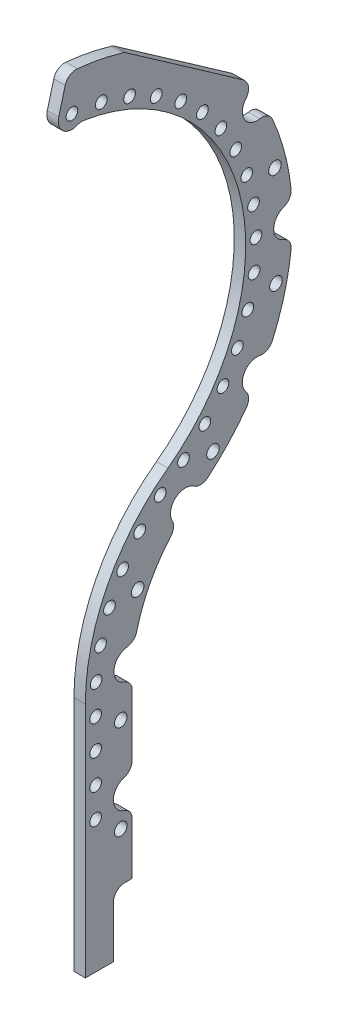
from build123d import *

# Parameters (mm, degrees)
SKETCH_3_R      = 1.025
SKETCH_3_R_2    = 1.1
EXTRUDE_1_DEPTH = 1
FILLET_R2_1_R   = 2


with BuildPart() as part:
    # 草图3 → 凸台-拉伸1 (new, symmetric)
    with BuildSketch(Plane(origin=(0, 0, 0), x_dir=(0, 0, -1), z_dir=(1, 0, 0))):
        with BuildLine():
            Line((17.7, -14.496003195), (17.7, -0.091005487))
            ThreePointArc((17.7, -0.091005487), (14.516449024, 2.667043271), (18.130694373, 4.830156842))
            ThreePointArc((18.130694373, 4.830156842), (20.784604254, 12.605737141), (25.63176658, 19.239582485))
            ThreePointArc((25.63176658, 19.239582485), (25.323964311, 23.435289305), (29.409373215, 22.431231514))
            ThreePointArc((29.409373215, 22.431231514), (34.557047376, 27.097753162), (38.858437765, 32.554218527))
            ThreePointArc((38.858437765, 32.554218527), (37.328835208, 36.351942354), (41.382561796, 36.926129595))
            ThreePointArc((41.382561796, 36.926129595), (44.352566659, 44.759188173), (45.696996288, 53.027818322))
            ThreePointArc((45.696996288, 53.027818322), (42.473459702, 55.551942354), (45.696996288, 58.076066385))
            ThreePointArc((45.696996288, 58.076066385), (44.352566659, 66.344696534), (41.382561796, 74.177755113))
            ThreePointArc((41.382561796, 74.177755113), (37.328835208, 74.751942354), (38.858437765, 78.54966618))
            ThreePointArc((38.858437765, 78.54966618), (38.104416138, 79.651403013), (37.315512578, 80.728437754))
            Line((37.315512578, 80.728437754), (16.362174958, 95.400122706))
            ThreePointArc((16.362174958, 95.400122706), (11.434946284, 96.597021417), (6.398875236, 97.187053049))
            Line((6.398875236, 97.187053049), (4.831835438, 91.338780905))
            ThreePointArc((4.831835438, 91.338780905), (5.775264763, 88.750397581), (8.530219021, 88.754160598))
            ThreePointArc((8.530219021, 88.754160598), (36.525725618, 63.864609611), (23.943591586, 28.581071791))
            ThreePointArc((23.943591586, 28.581071791), (13.315993793, 16.011675448), (9.5, 0))
            Line((9.5, 0), (9.5, -41.5))
            Line((9.5, -41.5), (14.4, -41.5))
            Line((14.4, -41.5), (14.4, -30.5))
            Line((14.4, -30.5), (17.7, -30.5))
            Line((17.7, -30.5), (17.7, -19.503996805))
            ThreePointArc((17.7, -19.503996805), (14.4, -17), (17.7, -14.496003195))
        make_face()
        with Locations((11.3, -18.362276)):
            Circle(SKETCH_3_R, mode=Mode.SUBTRACT)
        with Locations((15.7, -22)):
            Circle(SKETCH_3_R_2, mode=Mode.SUBTRACT)
        with Locations((15.7, -5.5)):
            Circle(SKETCH_3_R_2, mode=Mode.SUBTRACT)
        with Locations((18.656131285, 12.825388146)):
            Circle(SKETCH_3_R_2, mode=Mode.SUBTRACT)
        with Locations((42.693459702, 64.748985357)):
            Circle(SKETCH_3_R_2, mode=Mode.SUBTRACT)
        with Locations((31.841454389, 27.178918703)):
            Circle(SKETCH_3_R_2, mode=Mode.SUBTRACT)
        with Locations((42.866043117, 47.112423882)):
            Circle(SKETCH_3_R_2, mode=Mode.SUBTRACT)
        with Locations((7.150057421, 90.717615196)):
            Circle(SKETCH_3_R, mode=Mode.SUBTRACT)
        with Locations((12.2828186, 89.884090939)):
            Circle(SKETCH_3_R, mode=Mode.SUBTRACT)
        with Locations((17.237437698, 88.305563273)):
            Circle(SKETCH_3_R, mode=Mode.SUBTRACT)
        with Locations((21.90640009, 86.016286055)):
            Circle(SKETCH_3_R, mode=Mode.SUBTRACT)
        with Locations((26.188389865, 83.065936319)):
            Circle(SKETCH_3_R, mode=Mode.SUBTRACT)
        with Locations((29.990488371, 79.518536292)):
            Circle(SKETCH_3_R, mode=Mode.SUBTRACT)
        with Locations((33.230190537, 75.451064119)):
            Circle(SKETCH_3_R, mode=Mode.SUBTRACT)
        with Locations((35.837195224, 70.951783448)):
            Circle(SKETCH_3_R, mode=Mode.SUBTRACT)
        with Locations((37.75493075, 66.118328115)):
            Circle(SKETCH_3_R, mode=Mode.SUBTRACT)
        with Locations((38.94178249, 61.055583509)):
            Circle(SKETCH_3_R, mode=Mode.SUBTRACT)
        with Locations((39.371995907, 55.873410565)):
            Circle(SKETCH_3_R, mode=Mode.SUBTRACT)
        with Locations((39.036235422, 50.684261801)):
            Circle(SKETCH_3_R, mode=Mode.SUBTRACT)
        with Locations((37.941786997, 45.600741107)):
            Circle(SKETCH_3_R, mode=Mode.SUBTRACT)
        with Locations((36.112400028, 40.733160259)):
            Circle(SKETCH_3_R, mode=Mode.SUBTRACT)
        with Locations((33.587771989, 36.187145162)):
            Circle(SKETCH_3_R, mode=Mode.SUBTRACT)
        with Locations((30.422686996, 32.061343787)):
            Circle(SKETCH_3_R, mode=Mode.SUBTRACT)
        with Locations((26.685827006, 28.445285516)):
            Circle(SKETCH_3_R, mode=Mode.SUBTRACT)
        with Locations((22.623630861, 25.1989703)):
            Circle(SKETCH_3_R, mode=Mode.SUBTRACT)
        with Locations((19.013334846, 21.456542922)):
            Circle(SKETCH_3_R, mode=Mode.SUBTRACT)
        with Locations((16.021763505, 17.203249973)):
            Circle(SKETCH_3_R, mode=Mode.SUBTRACT)
        with Locations((13.7201441, 12.54035944)):
            Circle(SKETCH_3_R, mode=Mode.SUBTRACT)
        with Locations((12.163276612, 7.57889155)):
            Circle(SKETCH_3_R, mode=Mode.SUBTRACT)
        with Locations((11.388228987, 2.43697545)):
            Circle(SKETCH_3_R, mode=Mode.SUBTRACT)
        with Locations((11.3, -2.762276)):
            Circle(SKETCH_3_R, mode=Mode.SUBTRACT)
        with Locations((11.3, -7.962276)):
            Circle(SKETCH_3_R, mode=Mode.SUBTRACT)
        with Locations((11.3, -13.162276)):
            Circle(SKETCH_3_R, mode=Mode.SUBTRACT)
    extrude(amount=EXTRUDE_1_DEPTH, both=True)

    # R2 圆角1
    fillet_r2_1_edges = [part.edges().sort_by_distance(p)[0] for p in [
        (0, 19.239582485, -25.63176658),
        (0, 4.830156842, -18.130694373),
        (0, -0.091005487, -17.7),
        (0, -14.496003195, -17.7),
        (0, -19.503996805, -17.7),
        (0, -30.5, -14.4),
        (0, 88.754160598, -8.530219021),
        (0, 97.187053049, -6.398875236),
        (0, 95.400122706, -16.362174958),
        (0, 80.728437754, -37.315512578),
        (0, 78.54966618, -38.858437765),
        (0, 74.177755113, -41.382561796),
        (0, 58.076066385, -45.696996288),
        (0, 53.027818322, -45.696996288),
        (0, 36.926129595, -41.382561796),
        (0, 32.554218527, -38.858437765),
        (0, 22.431231514, -29.409373215),
    ]]
    fillet(fillet_r2_1_edges, radius=FILLET_R2_1_R)


solid = part.part
